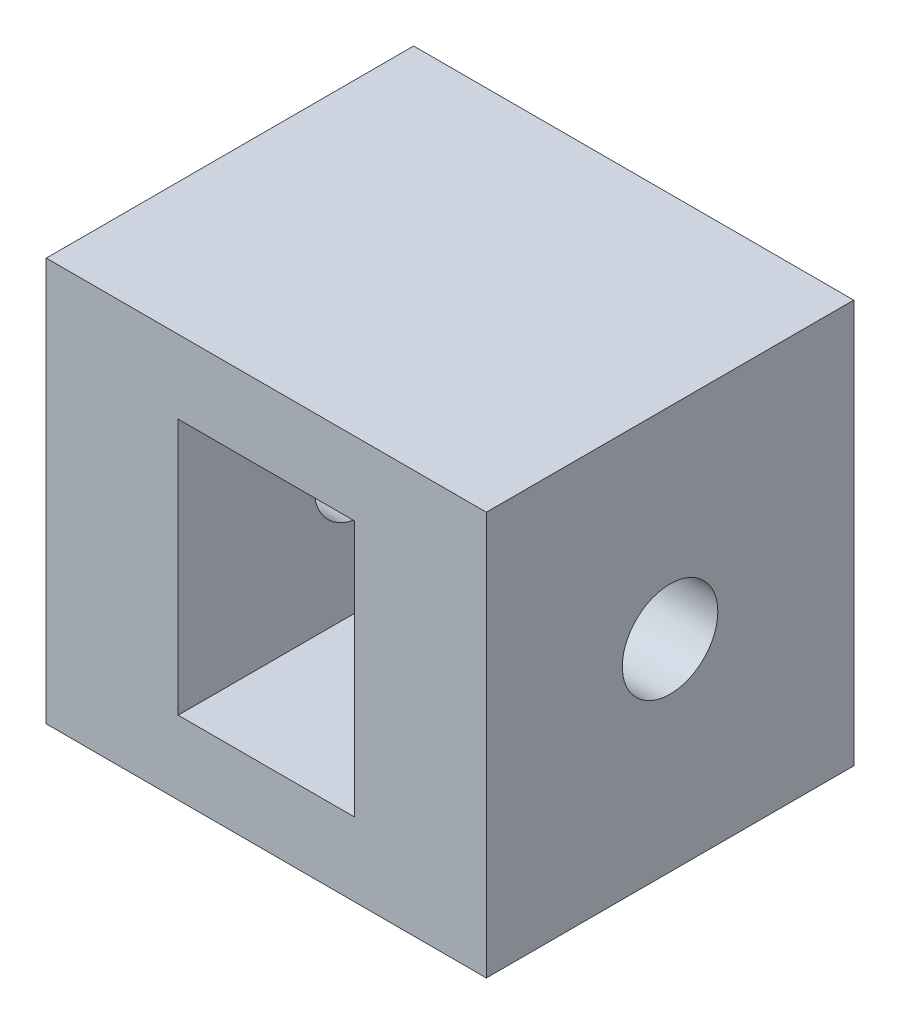
SolidWorks part; units mm, degrees
ref_plane "Front Plane" through (0, 0, 0) normal (0, 0, 1) x (1, 0, 0)
ref_plane "Top Plane" through (0, 0, 0) normal (0, 1, 0) x (1, 0, 0)
ref_plane "Right Plane" through (0, 0, 0) normal (1, 0, 0) x (0, 0, -1)
sketch "Sketch1" plane through (0, 0, 0) normal (0, 0, 1) x (1, 0, 0)
  line L0 (-2, 8.98) -> (6.39, 8.98)
  line L1 (1.59, 0) -> (4.8, 0)
  line L3 (1.59, 6.98) -> (4.8, 6.98)
  line L6 (-2, -2) -> (6.39, -2)
  line L7 (-2, -2) -> (-2, 8.98)
  line L8 (4.8, 6.98) -> (6.39, 6.98)
  line L9 (1.59, 3.49) -> (1.59, 6.98)
  line L10 (1.59, 3.49) -> (1.59, 0)
  line L11 (0, 6.98) -> (4.8, 6.98) construction
  line L12 (0, 0) -> (0, 6.98) construction
  line L13 (0, 0) -> (4.8, 0) construction
  line L14 (6.39, 6.98) -> (6.39, 0)
  line L16 (6.39, 0) -> (4.8, 0)
  line L17 (-2, 8.98) -> (6.8, 8.98) construction
  line L18 (4.8, 0) -> (4.8, 6.98) construction
  line L19 (6.8, -2) -> (6.8, 8.98) construction
  line L20 (-2, -2) -> (6.8, -2) construction
  line L21 (6.39, 8.98) -> (9.98, 8.98)
  line L22 (9.98, 8.98) -> (9.98, -2)
  line L23 (9.98, -2) -> (6.39, -2)
  dimension "D1" = 3.59
  dimension "D2" = 6.98
  dimension "D3" = 2
extrude "Boss-Extrude1" add sketch "Sketch1" along normal blind 10
sketch "Sketch4" plane through (9.98, 0, 0) normal (1, 0, 0) x (0, 0, -1)
  circle A0 centre (-5, 3.49) radius 1.3
extrude "Cut-Extrude2" cut sketch "Sketch4" against normal through all
